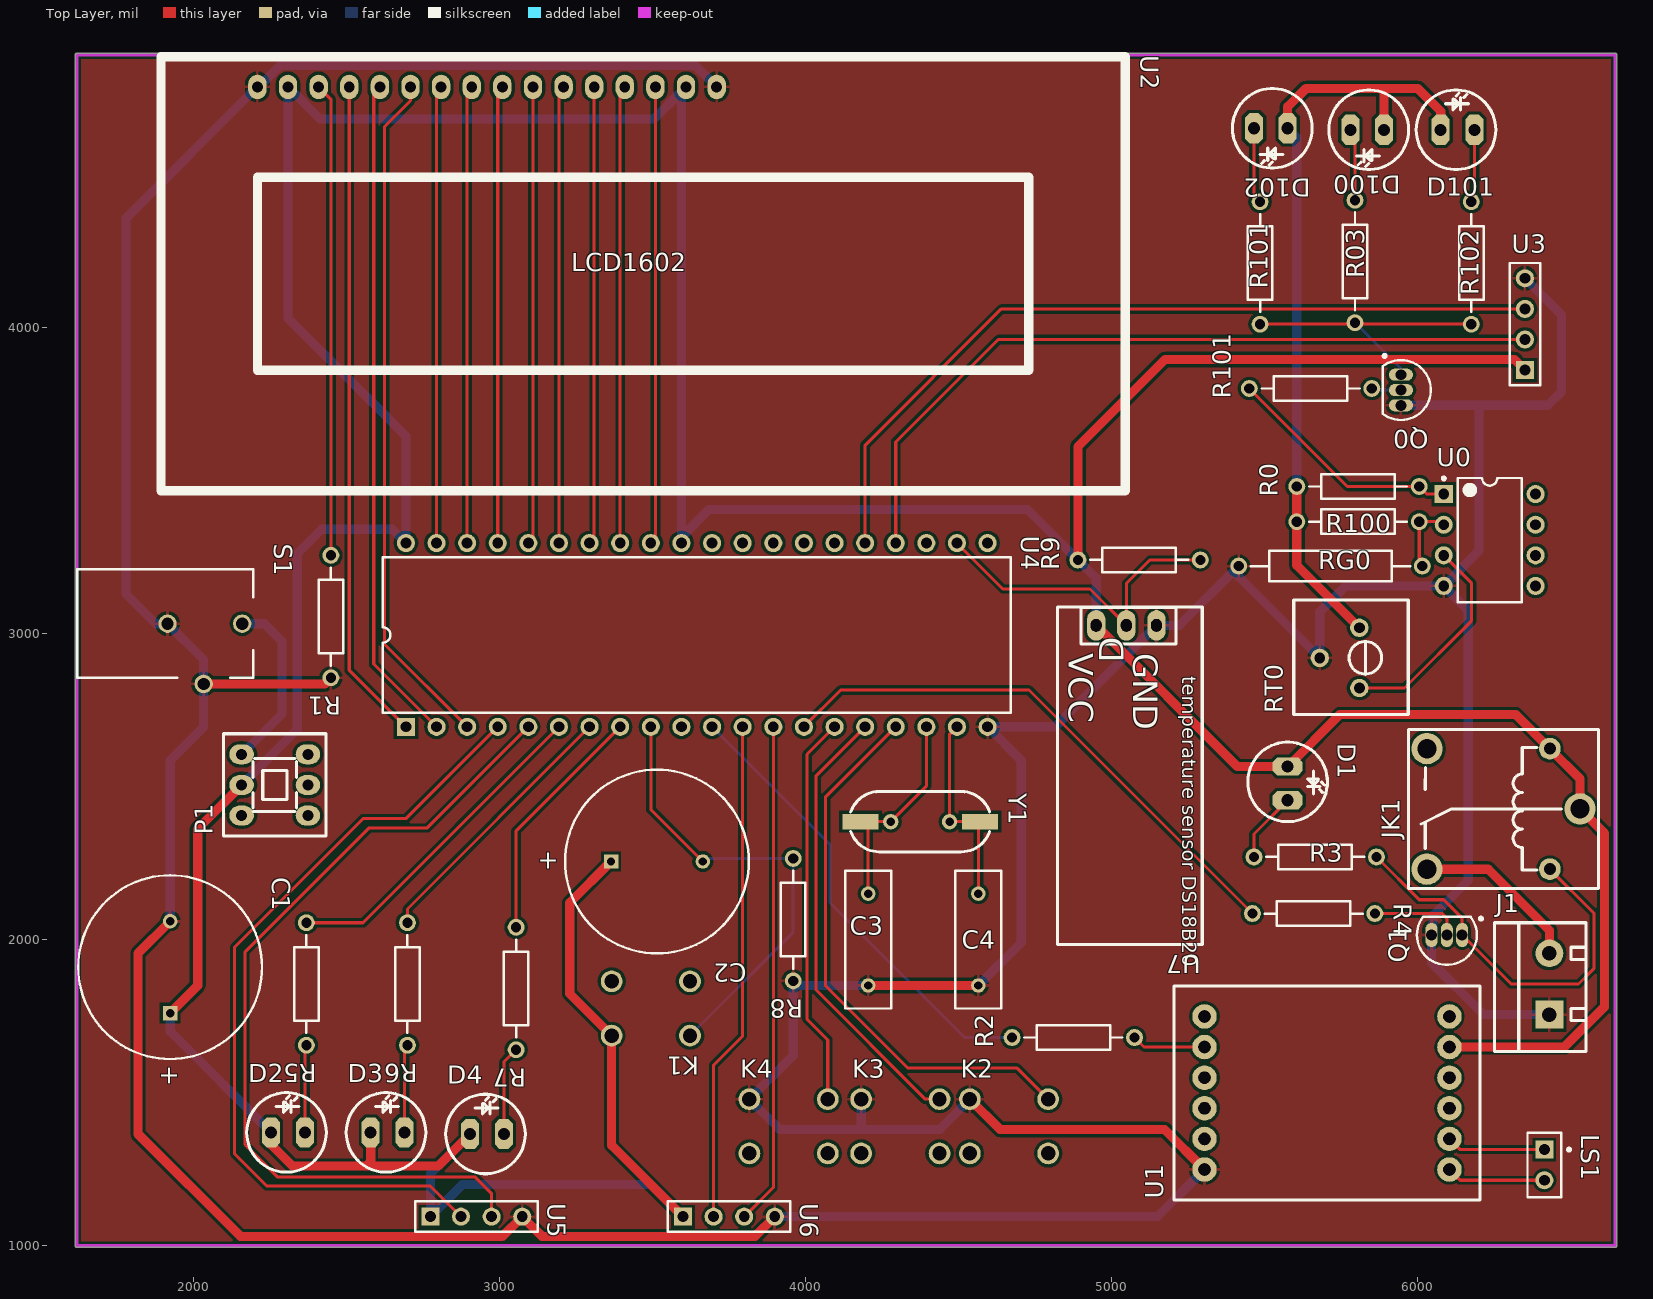
[diagram p0: Top Layer view]
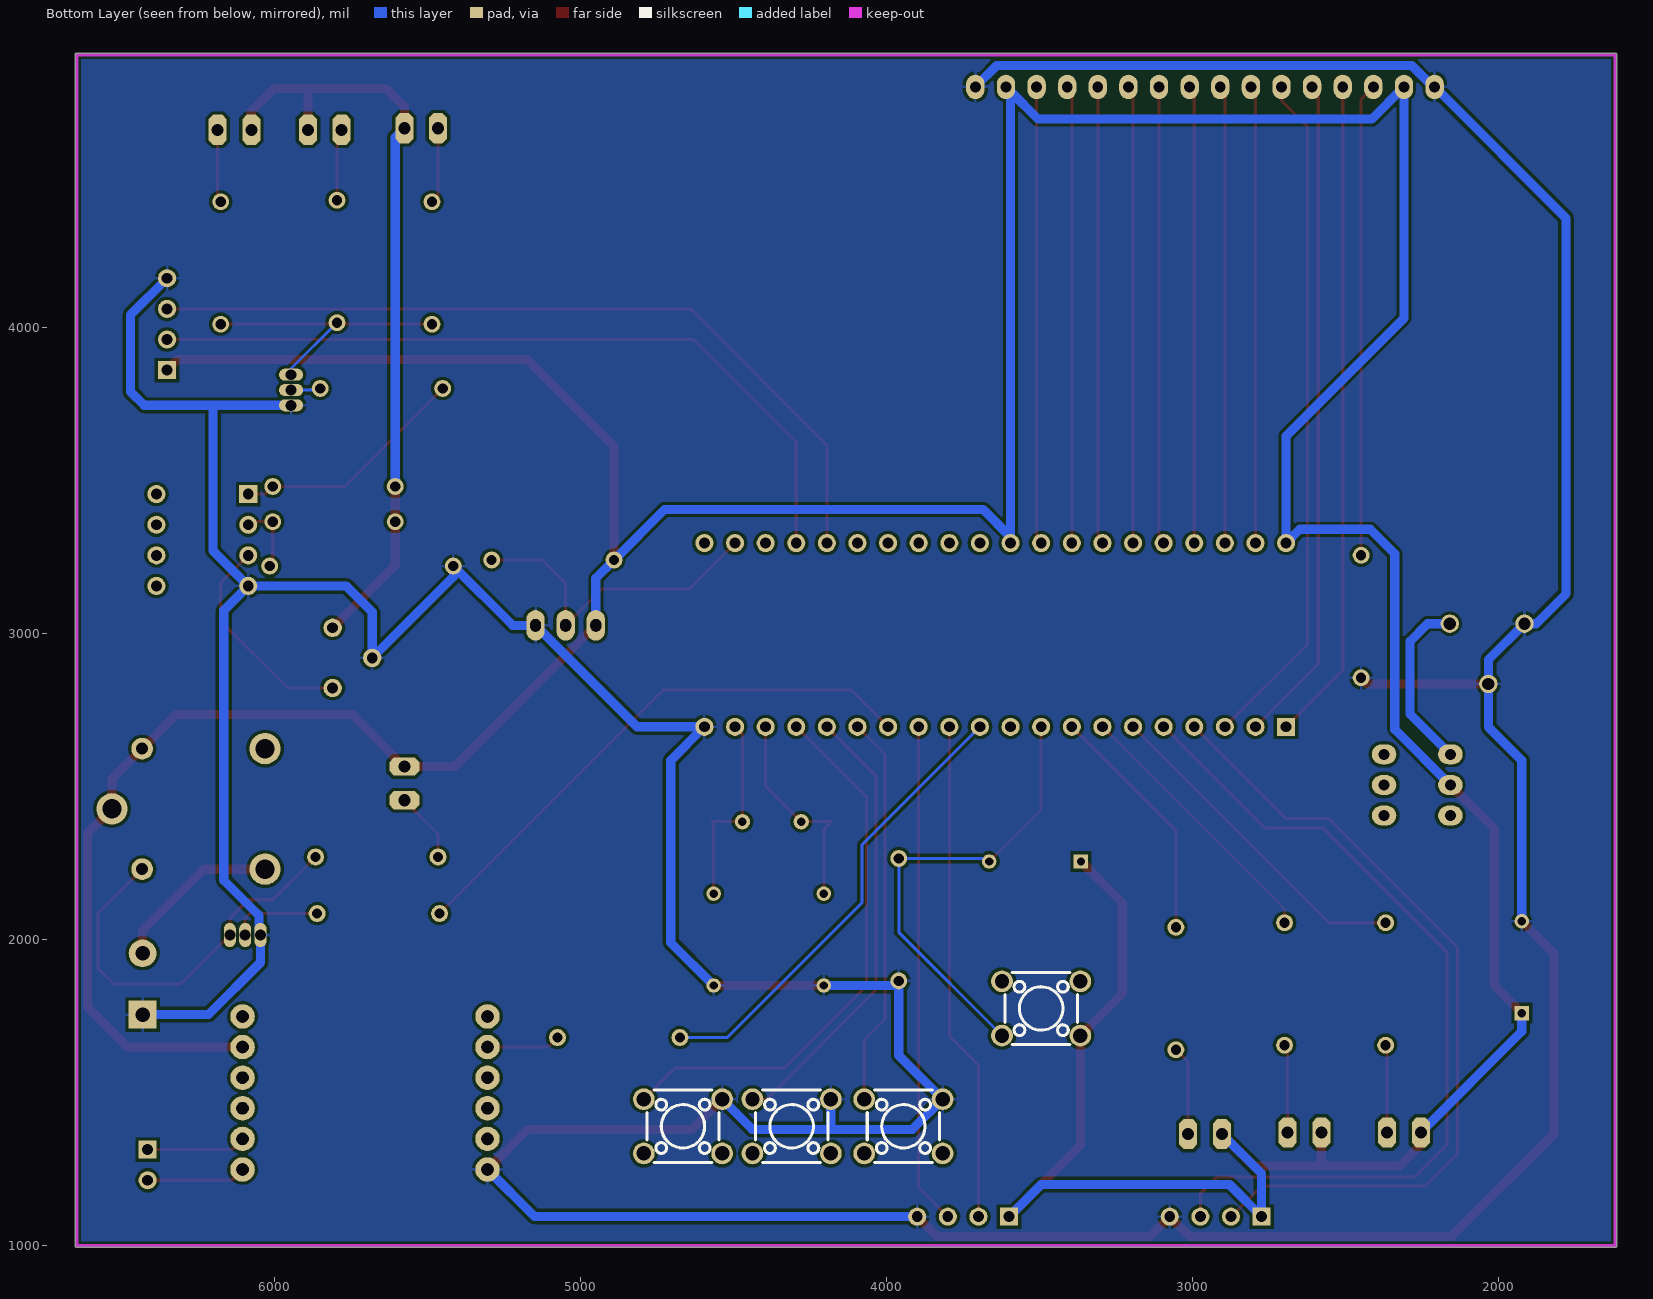
[diagram p1: Bottom Layer view, seen from below]
# Altium PCB MISC80724.PcbDoc
Units mil, origin at the board's own origin, x right, y up, seen from the top; angles counter-clockwise.
Board outline 5035.03 x 3900.03 mil, 2 copper layers (Top Layer, Bottom Layer); 48 components, 52 nets, 198 pads, 0 vias.

## Layer stack, top to bottom (the 12.6 mil dielectric is the usual default, probably not edited)
Top Solder: solder mask 0.4, Solder Resist, Dk 3.5
Top Layer: signal copper 1.4
Dielectric 1: dielectric 12.6, FR-4, Dk 4.8
Bottom Layer: signal copper 1.4
Bottom Solder: solder mask 0.4, Solder Resist, Dk 3.5

## Board outline
1614.98,1000 ccw(c1620,1000) 1620,994.99 6645,994.99 ccw(c6645,1000) 6650.02,1000 6650.02,4890 ccw(c6645,4890) 6645,4895.02 1620,4895.02 ccw(c1620,4890) 1614.98,4890

## Design rules (kind name [scope] priority, off if disabled: settings)
Clearance [All] p1: gap=10 ignorepadtopadclearanceinfootprint=TRUE except(0: Arc-Hole Track-Hole SMDPad-Hole THPad-Hole Via-Hole Fill-Hole Poly-Hole Region-Hole Text-Hole)
MinimumSolderMaskSliver [All] p1: minsoldermaskwidth=0
PolygonConnect [All] p1: connectstyle=Relief reliefconductorwidth=10 reliefentries=4 polygonreliefangle="90 Angle" airgapwidth=10
RoutingVias [All] p1: holewidth=28 width=50 viastyle="Through Hole" minholewidth=28 minwidth=50 maxholewidth=28 maxwidth=50
SilkToSilkClearance [All] p1: silktosilkclearance=0
SilkToSolderMaskClearance [IsPad] p1: minsilkscreentomaskgap=0 clearancetoexposedcopper=TRUE
SolderMaskExpansion [All] p1: expansion=4
Width [All] p1: maxlimit=30 minlimit=10 preferedwidth=10
27 further rules are at their usual default settings.

## Components (designator, comment, footprint, x,y, rotation, side; value= is the part's Value field where it differs from the comment)
C1 "470uf" RB7.6-15 1925,1910 r270 top
C2 "10uf" RB7.6-15 3515,2255 r180 top
C3 "22PF" RAD-0.3 4205,2000 r90 top
C4 "22PF" RAD-0.3 4565,2000 r90 top
D1 "LED-R" LED 5575,2565 r270 top
D2 "LED-G" LED 2255,1370 r0 top
D3 "LED-R" LED 2580,1370 r0 top
D4 "LED-Y" LED 2905,1365 r0 top
D100 "white LED" LED 5890,4645 r180 top
D101 "white LED" LED 6075,4645 r0 top
D102 "white LED" LED 5575,4650 r180 top
J1 "" KF301-5.0-2P 6430,1755 r90 top
JK1 "HFKW-012-1ZW" 012-1ZW_W 6530,2426.85 r180 top
K1 "push button" 四脚轻触开关 3495,1775 r180 top
K2 "push button" 四脚轻触开关 4665,1390 r0 top
K3 "push button" 四脚轻触开关 4310,1390 r0 top
K4 "push button" 四脚轻触开关 3945,1390 r0 top
LS1 "passive buzzer" PIN2 6413.48,1313.94 r270 top
P1 "latching switch" 自锁开关 2266.73,2505 r90 top
Q0 "9012" TO-92A 5945,3795 r180 top
Q1 "9012" TO-92A 6095,2015 r90 top
R0 "10K" AXIAL-0.4 5805,3480 r180 top
R1 "2K" AXIAL-0.4 2450,3055 r270 top
R2 "1K" AXIAL-0.4 4875,1680 r180 top
R03 "1K" AXIAL-0.4 5795,4215 r90 top
R3 "1K" AXIAL-0.4 5665,2270 r0 top
R4 "1K" AXIAL-0.4 5660,2085 r0 top
R5 "1K" AXIAL-0.4 2370,1855 r270 top
R6 "1K" AXIAL-0.4 2700,1855 r270 top
R7 "1K" AXIAL-0.4 3055,1840 r270 top
R8 "10K" AXIAL-0.4 3960,2065 r270 top
R9 "10K" AXIAL-0.4 5090,3240 r180 top
R100 "10K" AXIAL-0.4 5805,3365 r180 top
R101 "1K" AXIAL-0.4 5650,3800 r180 top
R101 "1K" AXIAL-0.4 5485,4210 r90 top
R102 "1K" AXIAL-0.4 6175,4210 r90 top
RG0 "photoresistor" AXIAL-0.6 5715,3220 r0 top
RT0 "10K" 电位器 5794.1,2922.01 r90 top
S1 "" KLD-0202 1620.98,3031.85 r0 top
U0 "LM393" DIP-8 6235,3305 r0 top
U1 "voice playback module-MY1680" MY1680 5703.48,1498.94 r180 top
U2 "LCD1602" LCD1602 2210,4785 r0 top
U3 "ultrasonic module" HDR1X4 6350,3860 r90 top
U4 "STC89C52" DIP-40 3645,2995 r0 top
U5 "ultrasonic module" HDR1X4 2775,1095 r0 top
U6 "ultrasonic module" HDR1X4 3600,1095 r0 top
U7 "DS18B20" DS18B20 5060,2535 r270 top
Y1 "11.0592MHz" XTAL_US 4278.82,2385 r0 top

## Footprints (in the part's own frame and the unit in brackets; to place one, negate y for a bottom-side part, rotate by r counter-clockwise, add the part's x,y. Pads: shape width x height; smd on the part's side, far side on the other; paste and mask are expansions set on the pad)
012-1ZW_W [mm] "单刀双投"
  round 1.8 hole 1: 1(2.5,5) 2(2.5,-5)
  round 2.6 hole 1.6: 3(0,0) 4(12.7,5) 5(12.7,-5)
  silkscreen extent -1.52,-6.6 14.22,6.6, body extent -1.52,-6.1 13.98,6.1, height 12.9
AXIAL-0.4 [mm] "Axial Device, Thru-Hole; 2 Leads; 0.4 in Pin Spacing"
  round 1.4 hole 0.85: 1(-5.08,0) 2(5.08,0)
  silkscreen extent -4.06,-1.02 4.06,1.02
AXIAL-0.6 [mm] "Axial Device, Thru-Hole; 2 Leads; 0.6 in Pin Spacing"
  round 1.4 hole 0.85: 1(-7.62,0) 2(7.62,0)
  silkscreen extent -6.6,-1.27 6.6,1.27
DIP-8 [mm] "DIP; 8 Leads; Row Spacing 7.62 mm; Pitch 2.54 mm"
  rect 1.5x1.5 hole 0.9: 1(-3.81,3.81)
  round 1.5 hole 0.9: 2(-3.81,1.27) 3(-3.81,-1.27) 4(-3.81,-3.81) 5(3.81,-3.81) 6(3.81,-1.27) 7(3.81,1.27) 8(3.81,3.81)
  silkscreen extent -3.93,-5.15 2.65,5.23, body extent -3.6,-5.15 3.6,5.15, height 5.08
DIP-40 [mm]
  rect 1.5x1.5 hole 0.9: 1(-24.13,-7.62)
  round 1.5 hole 0.9: 2(-21.59,-7.62) 3(-19.05,-7.62) 4(-16.51,-7.62) 5(-13.97,-7.62) 6(-11.43,-7.62) 7(-8.89,-7.62) 8(-6.35,-7.62) 9(-3.81,-7.62) 10(-1.27,-7.62) 11(1.27,-7.62) 12(3.81,-7.62) 13(6.35,-7.62) 14(8.89,-7.62) 15(11.43,-7.62) 16(13.97,-7.62) 17(16.51,-7.62) 18(19.05,-7.62) 19(21.59,-7.62) 20(24.13,-7.62) 21(24.13,7.62) 22(21.59,7.62) 23(19.05,7.62) 24(16.51,7.62) 25(13.97,7.62) 26(11.43,7.62) 27(8.89,7.62) 28(6.35,7.62) 29(3.81,7.62) 30(1.27,7.62) 31(-1.27,7.62) 32(-3.81,7.62) 33(-6.35,7.62) 34(-8.89,7.62) 35(-11.43,7.62) 36(-13.97,7.62) 37(-16.51,7.62) 38(-19.05,7.62) 39(-21.59,7.62) 40(-24.13,7.62)
  silkscreen extent -26.05,-6.45 26.05,6.45
DS18B20 [mil]
  oval 99.37x60 hole 35.43 slot 41.34 at 0 deg paste+0 mask+4: 1(-491.35,86.55) 2(-491.35,-11.88) 3(-491.35,-110.3)
  silkscreen extent -551,-236 551,236
HDR1X4 [mm] "Connector; Header; 4 Position"
  rect 1.5x1.5 hole 0.9: 1(0,0)
  round 1.5 hole 0.9: 2(2.54,0) 3(5.08,0) 4(7.62,0)
  silkscreen extent -1.27,-1.27 8.89,1.27
KF301-5.0-2P [mm] "可拼接端子/6A"
  rect 2.3x2.3 hole 1.2: 1(0,0)
  round 2.3 hole 1.2: 2(5.08,0)
  silkscreen extent -3.05,-3.05 7.62,4.57, body extent -3,-3.09 7.5,4.51, height 10.05
KLD-0202 [mm] "DC Power Jack, 2.5mm, KLD Series, PCB Mount"
  round 1.524 hole 1.016: 1(13.7,0) 2(7.5,0) 3(10.5,-5)
  oval 0x1.5 all layers, no hole: 1A(13.7,-1.25) 1B(13.7,1.25) 3A(9.5,-5) 3B(11.5,-5)
  round 0 all layers, no hole: 2A(7.5,-1) 2B(7.5,1)
  silkscreen extent 0,-4.5 14.6,4.5
LCD1602 [mil]
  oval 60x80 hole 35.43: 1(0,0) 2(100,0) 3(200,0) 4(300,0) 5(400,0) 6(500,0) 7(600,0) 8(700,0) 9(800,0) 10(900,0) 11(1000,0) 12(1100,0) 13(1200,0) 14(1300,0) 15(1400,0) 16(1500,0)
  silkscreen extent -315,-1319 2835,98, body extent -315,-1357 2854,80, height 414
LED [mm]
  oct 1.5x2.5 hole 1: 1(0,0) 2(2.794,0)
  silkscreen extent -2.03,-3.3 4.57,3.3
MY1680 [mil]
  round 80 hole 40 slot 40.2 at 0 deg paste+0 mask+2: 1(-400,250) 2(-400,150) 3(-400,50) 4(-400,-50) 5(-400,-150) 6(-400,-250) 7(400,-250) 8(400,-150) 9(400,-50) 10(400,50) 11(400,150) 12(400,250)
  silkscreen extent -500,-350 500,350
PIN2 [mm] "Photosensitive Diode; 2 Leads"
  rect 1.5x1.5 hole 0.9: 1(0,0)
  round 1.5 hole 0.9: 2(2.54,0)
  silkscreen extent -1.4,-1.4 3.94,2.18
RAD-0.3 [mm] "Radial Cap, Thru-Hole; 2 Leads; 0.3 in Pin Spacing"
  round 1.2 hole 0.7: 1(-3.81,0) 2(3.81,0)
  silkscreen extent -5.71,-1.91 5.71,1.91
RB7.6-15 [mm] "Polarized Capacitor (Radial); 2 Leads"
  rect 1.2x1.2 hole 0.7: 1(3.81,0)
  round 1.2 hole 0.7: 2(-3.81,0)
  silkscreen extent -7.62,-7.62 7.62,7.62
TO-92A [mm] "TO, Flat Index; 3 In-Line, Axial Leads; Body Dia. 4.5mm; Leads 0.51 x 0.48 mm (max)"
  oval 2x1 hole 0.9: 1(0,-1.27) 2(0,0) 3(0,1.27)
  silkscreen extent -2.48,-2.95 1.5,2.48, body extent -2.48,-2.5 1.5,2.5, height 6.86
XTAL_US [mm]
  rect 3x1.27 smd: 1(-2.51,0) 2(7.39,0)
  round 1.27 hole 0.711: 1(0,0) 2(4.88,0)
  silkscreen extent -3.33,-2.5 8.21,2.5
四脚轻触开关 [mm]
  round 1.8 hole 1.2 paste+0 mask+0.102: 1(3.25,2.25) 2(-3.25,2.25) 3(3.25,-2.25) 4(-3.25,-2.25)
电位器 [mil]
  round 60 hole 35.43 paste+0 mask+2: 1(96.41,-15.12) 2(-2.01,114.1) 3(-100.44,-15.12)
  silkscreen extent -187,-175 187,199
自锁开关 [mil]
  oval 65x80 hole 36 paste+0 mask+4: 1(-100,-108.27) 2(0,-108.27) 3(100,-108.27) 4(-100,108.27) 5(0,108.27) 6(100,108.27)
  silkscreen extent -167,-167 167,167

## Part data
C1 C2: library part 电解电容
C3 C4: library part 瓷片电容
D1 D2 D3 D4 D100 D101 D102: library part LED-5MM
J1: library part 端子2P-5mm
JK1: "12V one-group changeover"
K1 K2 K3 K4: library part 按键
LS1: library part SPEAKER
P1: library part 自锁开关
Q0 Q1: library part PNP三极管
R0 R1 R03 R3 R4 R5 R6 R7 R8 R9 R100 R101 R101 R102: library part 电阻-定值
R2: library part RES2
RG0: library part 电阻-光敏
RT0: library part 电位器
S1: library part 电源接口-小
U1: library part Component_1
U3 U5 U6: library part 超声波模块
Y1: library part 晶振

## Nets (pads, with @x,y where several pads share a name; then routed paths per layer and width w, separated by ;. In a path a pad name is that pad's centre, name@x,y a point inside that pad or via, vN(x,y) a via of type N, cw(c..) or ccw(c..) an arc to the next point about the centre after c; other vN are vias at no path point)
5V: D100.1 D101.1 D102.1 R0.2 R100.2 RT0.1 | length 2549.5
  Top Layer w30: D102.1 5575,4720 5635,4780 5890,4780 ; R0.2 R100.2 5605,3222.64 RT0.1 ; D100.1 5890,4780 ; D101.1 6075,4705 6000,4780 5890,4780
  Bottom Layer w30: D102.1 5605,4620 R0.2
B0: U2.7 U4.39 | length 1496.2
  Top Layer w10: U4.39 2795,4770 U2.7
B1: U2.8 U4.38 | length 1496.2
  Top Layer w10: U4.38 2895,4770 U2.8
B2: U2.9 U4.37 | length 1496.2
  Top Layer w10: U4.37 2995,4770 U2.9
B3: U2.10 U4.36 | length 1496.2
  Top Layer w10: U4.36 3110,3310 U2.10
B4: U2.11 U4.35 | length 1496.2
  Top Layer w10: U4.35 3195,4770 U2.11
B5: U2.12 U4.34 | length 1496.2
  Top Layer w10: U4.34 3310,3310 U2.12
B6: U2.13 U4.33 | length 1496.2
  Top Layer w10: U4.33 3395,4770 U2.13
B7: U2.14 U4.32 | length 1496.2
  Top Layer w10: U4.32 3510,3310 U2.14
EN: U2.6 U4.3 | length 2237
  Top Layer w10: U2.6 2710,4740 2625,4655 2625,2965 U4.3
GND: C1.2 C3.1 C4.1 J1.1 K2.2 K3.2 K4.2 Q0.3 Q1.3 R1.2 R8.2 RG0.1 RT0.2 S1.2 S1.3 U0.4 U1.12 U2.1 U2.16 U3.4 U4.20 U5.4 U6.4 U7.1 | length 18739.9
  Top Layer w30: C1.2 1820,1955 1820,1365 2155,1030 3010,1030 U5.4 3140,1030 3835,1030 U6.4 ; S1.3 2430,2835 R1.2 ; C3.1 C4.1 ; K2.2 4635.63,1380 5172.42,1380 U1.12
  Bottom Layer w30: C1.2 1925,2585 2034.37,2694.37 S1.3 2034.37,2913.74 S1.2 1878.52,3031.85 1780.37,3130 1780.37,4355.37 U2.1 2215,4785 2285,4855 3640,4855 U2.16 ; U6.4 5149.54,1095 U1.12 ; K3.2 4182.05,1382.95 4185,1380 ; C3.1 3975,1850 R8.2 3960,1621.54 K4.2 3915.63,1380 4185,1380 ; K2.2 4438.46,1380 4185,1380 ; C4.1 4705,1990 4705,2585 U4.20 4815.2,2695 U7.1 5221.35,3026.35 RG0.1 5415,3185 RT0.2 5680,3070 5765,3155 U0.4 ; Q0.3 6205,3745 ; U3.4 6470,4040 6470,3790 6425,3745 6205,3745 ; J1.1 6215,1755 6045,1925 Q1.3 6050.31,2020.32 6050.31,2079.37 6165,2194.05 6165,3075 U0.4 ; U0.4 6200,3270 6200,3740 6205,3745
NetC2_2: C2.2 K1.2 R8.1 U4.9 | length 1527.8
  Top Layer w10: U4.9 3495,2425 C2.2
  Bottom Layer w10: K1.2 3960,2023.46 R8.1 3675,2265 C2.2
NetC3_2: C3.2 U4.18 Y1.1 | length 702.3
  Top Layer w10: C3.2 4205,2360 4180,2385 4278.82,2385 4395,2501.18 U4.18
NetC4_2: C4.2 U4.19 Y1.2 | length 655.8
  Top Layer w10: U4.19 4470.94,2670.94 4470.94,2385 4569.76,2385 4565,2380.24 C4.2
NetD1_2: D1.2 R3.1 | length 230.6
  Top Layer w10: R3.1 5465,2345 D1.2
NetD2_2: D2.2 R5.2 | length 287.1
  Top Layer w10: D2.2 2365,1650 R5.2
NetD3_2: D3.2 R6.2 | length 289.1
  Top Layer w10: D3.2 2690,1645 R6.2
NetD4_2: D4.2 R7.2 | length 291.6
  Top Layer w10: D4.2 3015,1600 R7.2
NetD100_2: D100.2 R03.2 | length 236.2
  Top Layer w10: D100.2 5795,4630 R03.2
NetD101_2: D101.2 R102.2 | length 239.1
  Top Layer w10: R102.2 6185,4420 D101.2
NetD102_2: D102.2 R101.2@5485,4410 | length 248.3
  Top Layer w10: D102.2 5465,4430 R101.2@5485,4410
NetJ1_2: J1.2 JK1.4 | length 557.8
  Top Layer w30: JK1.4 6230,2230 6430,2030 J1.2
NetJK1_1: JK1.1 Q1.1 R3.2 | length 1319.2
  Top Layer w10: R3.2 6005,2130 6085,2130 6145,2070 Q1.1 6305,1855 6525,1855 6575,1905 6575,2086.57 JK1.1
NetLS1_1: LS1.1 U1.2 | length 324.5
  Top Layer w10: U1.2 6138.48,1313.94 LS1.1
NetLS1_2: LS1.2 U1.1 | length 324.5
  Top Layer w10: U1.1 6138.48,1213.94 LS1.2
NetP1_6: P1.6 S1.1 | length 577.7
  Bottom Layer w30: P1.6 2290,2736.54 2290,2975 2233.15,3031.85 S1.1
NetQ0_1: Q0.1 R03.1 R101.1@5485,4010 R102.1 | length 922.1
  Top Layer w10: R101.1@5485,4010 R102.1
  Bottom Layer w10: R03.1 5945,3865 Q0.1
NetQ0_2: Q0.2 R101.1@5850,3800 | length 97.1
  Bottom Layer w10: R101.1@5850,3800 5855,3795 Q0.2
NetQ1_2: Q1.2 R4.2 | length 296.2
  Top Layer w10: R4.2 6080,2085 6095,2070 Q1.2
NetR1_1: R1.1 U2.3 | length 1546.6
  Top Layer w10: U2.3 2450,4745 R1.1
NetR2_1: R2.1 U1.8 | length 241.3
  Top Layer w10: R2.1 5106.06,1648.94 U1.8
NetR100_1: R100.1 RG0.2 U0.2 | length 233.3
  Top Layer w10: RG0.2 6005,3230 R100.1 6075,3365 U0.2
NetRT0_3: RT0.3 U0.3 | length 708.5
  Top Layer w10: RT0.3 5956.57,2821.57 6175,3040 6175,3165 U0.3
OUT1: R0.1 R101.2@5450,3800 U0.1 | length 777.9
  Top Layer w10: R101.2@5450,3800 5770,3480 R0.1 6030,3455 U0.1
P13: U4.4 U5.2 | length 2658.1
  Top Layer w10: U5.2 2775,1195 2240,1195 2135,1300 2135,1975 2555,2395 2695,2395 U4.4
P14: U4.5 U5.3 | length 2805.7
  Top Layer w10: U5.3 2975,1170 2920,1225 2275,1225 2170,1330 2170,1960 2575,2365 2765,2365 U4.5
P15: R5.1 U4.6 | length 1090.1
  Top Layer w10: R5.1 2555,2055 U4.6
P16: R6.1 U4.7 | length 886.5
  Top Layer w10: R6.1 2700,2100 U4.7
P17: R7.1 U4.8 | length 795.8
  Top Layer w10: R7.1 3055,2355 U4.8
P21: R9.1 U4.22 U7.2 | length 1074.9
  Top Layer w10: U4.22 4645,3145 4929.47,3145 U7.2 5048.12,3163.12 5125,3240 R9.1
P23: U3.2 U4.24 | length 2523.8
  Top Layer w10: U4.24 4295,3625 4630,3960 U3.2
P24: U3.3 U4.25 | length 2659.3
  Top Layer w10: U4.25 4195,3615 4640,4060 U3.3
P31: R2.2 U4.11 | length 1511.7
  Bottom Layer w10: U4.11 4080,2310 4080,2120 4520,1680 R2.2
P32: U4.12 U6.2 | length 1639.4
  Top Layer w10: U6.2 3700,1590 3795,1685 U4.12
P33: U4.13 U6.3 | length 1639.4
  Top Layer w10: U6.3 3895,1190 U4.13
P34: R4.1 U4.14 | length 1817.1
  Top Layer w10: U4.14 4115,2815 4730,2815 R4.1
P35: K4.1 U4.15 | length 1281.8
  Top Layer w10: K4.1 4072.95,1672.05 4005,1740 4005,2605 U4.15
P36: K3.1 U4.16 | length 1476.9
  Top Layer w10: U4.16 4035,2535 4035,1835 4391.42,1478.58 K3.1
P37: K2.1 U4.17 | length 1822.1
  Top Layer w10: U4.17 4065,2465 4065,1850 4335,1580 4691.54,1580 K2.1
RS: U2.4 U4.1 | length 2166.6
  Top Layer w10: U2.4 2510,2880 U4.1
RW: U2.5 U4.2 | length 2183.2
  Top Layer w10: U2.5 2590,4765 2590,2900 U4.2
VCC: C1.1 C2.1 D1.1 D2.1 D3.1 D4.1 JK1.2 JK1.3 K1.1 P1.5 R9.2 U1.5 U2.2 U2.15 U3.1 U4.31 U4.40 U5.1 U6.1 U7.3 | length 17470
  Top Layer w30: C1.1 2015,1850 2015,2361.54 P1.5 ; D2.1 2255,1330 2325,1260 2565,1260 ; D3.1 2580,1275 2565,1260 ; D4.1 2800,1260 2565,1260 ; C2.1 3230,2120 3230,1823.46 K1.1 3367.05,1327.95 U6.1 ; R9.2 4890,3610 5175,3895 6315,3895 U3.1 ; U7.3 5411.05,2565 D1.1 5745,2735 6320.28,2735 JK1.2 6530,2525.28 JK1.3 6610,2346.85 6610,1780 6478.94,1648.94 U1.5
  Bottom Layer w30: C1.1 1925,1700 D2.1 ; P1.5 2340,2686.54 2340,3260 2420,3340 2650,3340 U4.40 2695,3645 2310,4030 U2.2 2415,4680 3505,4680 U2.15@3595,4770 ; D4.1 2775,1235 U5.1 2880,1200 3495,1200 U6.1 ; U4.31 U4.31@3595,3315 ; U2.15 U2.15@3595,4770 ; U7.3 4949.7,3180.3 R9.2 4725,3405 3685,3405 U4.31@3595,3315 ; U4.31@3595,3315 U2.15@3595,4770
pads on no net: JK1.5 K1.3 K1.4 K2.3 K2.4 K3.3 K3.4 K4.3 K4.4 P1.1 P1.2 P1.3 P1.4 S1.1A S1.1B S1.2A S1.2B S1.3A S1.3B U0.5 U0.6 U0.7 U0.8 U1.3 U1.4 U1.6 U1.7 U1.9 U1.10 U1.11 U4.10 U4.21 U4.23 U4.26 U4.27 U4.28 U4.29 U4.30

## Polygon pours and split planes (outlines as drawn)
GND on Top Layer "Top Layer-No Net" (solid, remove dead copper, pour order 0): 1030,5230 1035,5235 7690,5235 7690,1280 7020,610 6990,640 1260,640
GND on Bottom Layer "Top Layer-No Net" (solid, remove dead copper, pour order 2): 1395,5055 6725,5055 6905,5235 6905,265 1270,265 1115,420

## Keep-outs
Keep-Out Layer:
  lines w10: 1620,3035 1620,4890 1885,4890 6530,4890 ; 1620,3045 1620,1000 6645,1000 6645,1012.07 6645,4890 6515,4890